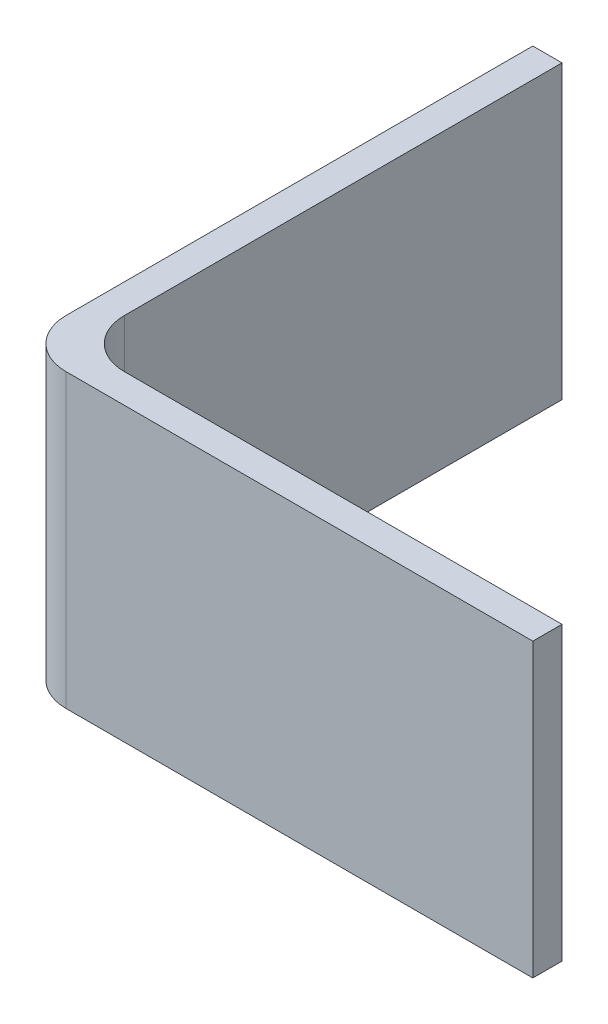
from build123d import *

# Parameters (mm, degrees)
BOSS_EXTRUDE1_DEPTH = 30


with BuildPart() as part:
    # Sketch1 → Boss-Extrude1 (new body)
    with BuildSketch(Plane(origin=(0, 0, 0), x_dir=(1, 0, 0), z_dir=(0, 1, 0))):
        with BuildLine():
            Line((5, 0), (50, 0))
            Line((50, 0), (50, -3))
            Line((50, -3), (2, -3))
            ThreePointArc((2, -3), (-1.535533906, -1.535533906), (-3, 2))
            Line((-3, 2), (-3, 50))
            Line((-3, 50), (0, 50))
            Line((0, 50), (0, 5))
            ThreePointArc((0, 5), (1.464466094, 1.464466094), (5, 0))
        make_face()
    extrude(amount=BOSS_EXTRUDE1_DEPTH)


solid = part.part
